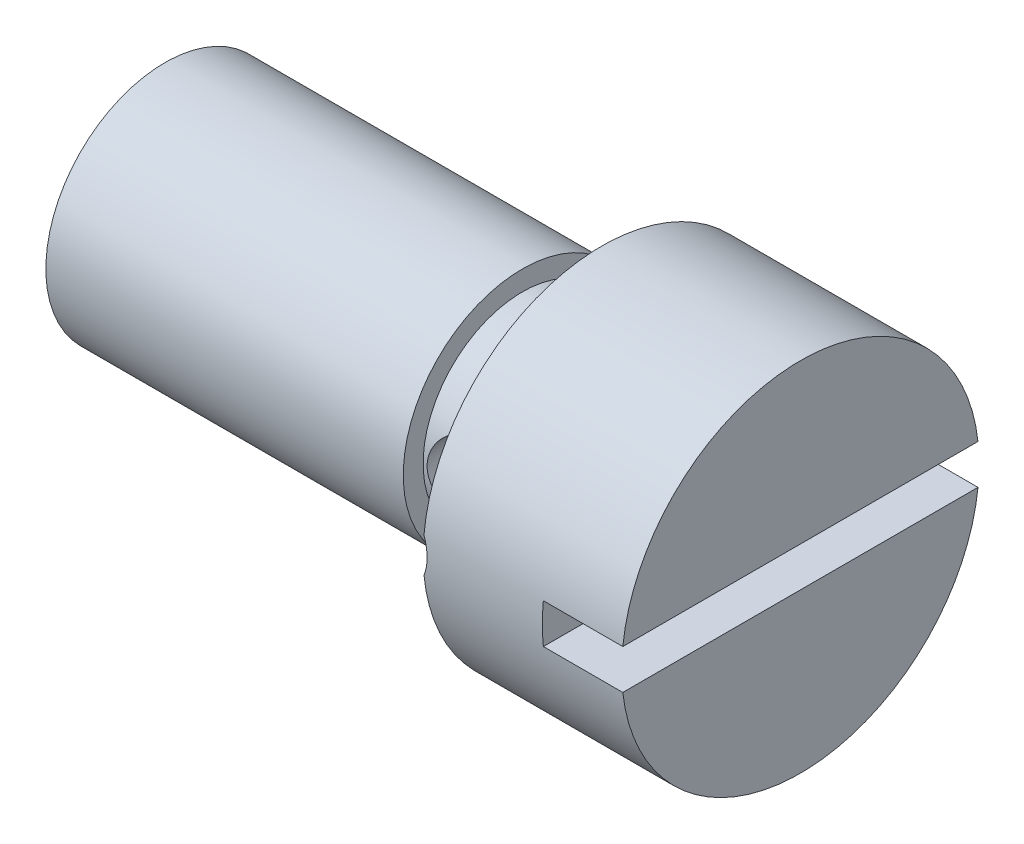
from build123d import *

# Parameters (mm, degrees)
SKETCH1_R               = 3
BOSS_EXTRUDE1_DEPTH     = 9
SKETCH2_R               = 2.5
BOSS_EXTRUDE2_DEPTH     = 2
SKETCH3_R               = 4.5
BOSS_EXTRUDE3_DEPTH     = 5
CUT_EXTRUDE1_DEPTH      = 18.219175358
CUT_EXTRUDE1_DEPTH_BACK = 10.1
SKETCH4_R               = 1
CUT_EXTRUDE2_DEPTH      = 18.219175358
CUT_EXTRUDE2_DEPTH_BACK = 18.219175358
SKETCH6_R               = 1
CUT_EXTRUDE3_DEPTH      = 18.219175503
CUT_EXTRUDE3_DEPTH_BACK = 18.219175503
SKETCH7_W               = 4
SKETCH7_H               = 1


with BuildPart() as part:
    # Sketch1 → Boss-Extrude1 (new body)
    with BuildSketch(Plane(origin=(0, 0, 0), x_dir=(0, 0, -1), z_dir=(1, 0, 0))):
        Circle(SKETCH1_R)
    extrude(amount=BOSS_EXTRUDE1_DEPTH)

    # Sketch2 → Boss-Extrude2 (add)
    with BuildSketch(Plane(origin=(9, 0, 0), x_dir=(0, 0, -1), z_dir=(1, 0, 0))):
        Circle(SKETCH2_R)
    extrude(amount=BOSS_EXTRUDE2_DEPTH)

    # Sketch3 → Boss-Extrude3 (add)
    with BuildSketch(Plane(origin=(11, 0, 0), x_dir=(0, 0, -1), z_dir=(1, 0, 0))):
        Circle(SKETCH3_R)
    extrude(amount=BOSS_EXTRUDE3_DEPTH)

    # Sketch4 → Cut-Extrude1 (cut, two sides: drawn at the far end of the back side and taken through both)
    with BuildSketch(Plane.ZY.offset(-CUT_EXTRUDE1_DEPTH_BACK)):
        with Locations(Location((0, 0, 0), (0, 0, 180))):
            Circle(SKETCH4_R)
    extrude(amount=CUT_EXTRUDE1_DEPTH + CUT_EXTRUDE1_DEPTH_BACK, mode=Mode.SUBTRACT)

    # Sketch6 → Cut-Extrude2 (cut, two sides: drawn at the far end of the back side and taken through both)
    with BuildSketch(Plane.XY.offset(-CUT_EXTRUDE2_DEPTH_BACK)):
        with Locations(Location((10.1, 0, 0), (0, 0, 334.158067237))):
            Circle(SKETCH6_R)
    extrude(amount=CUT_EXTRUDE2_DEPTH + CUT_EXTRUDE2_DEPTH_BACK, mode=Mode.SUBTRACT)

    # Sketch7 → Cut-Extrude3 (cut, two sides: drawn at the far end of the back side and taken through both)
    with BuildSketch(Plane.XY.offset(-CUT_EXTRUDE3_DEPTH_BACK)):
        with Locations((16, 0)):
            Rectangle(SKETCH7_W, SKETCH7_H)
    extrude(amount=CUT_EXTRUDE3_DEPTH + CUT_EXTRUDE3_DEPTH_BACK, mode=Mode.SUBTRACT)


solid = part.part
